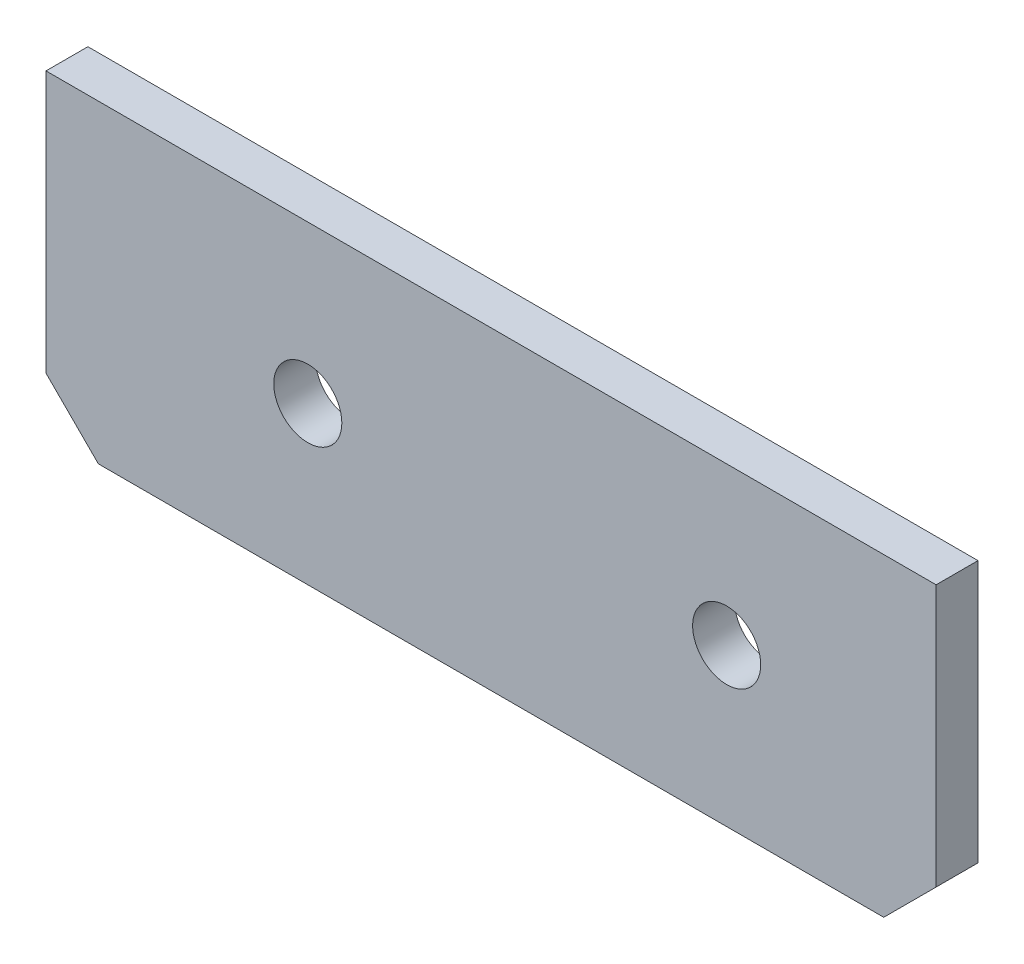
from build123d import *

# Parameters (mm, degrees)
EXTRUDE_1_DEPTH     = 8
SKETCH_2_R          = 6.5
CUT_EXTRUDE_1_DEPTH = 8


with BuildPart() as part:
    # 草图1 → 凸台-拉伸1 (new body)
    with BuildSketch(Plane.XY):
        Polygon((10, 0), (160, 0), (170, 10), (170, 60), (0, 60), (0, 10), align=None)
    extrude(amount=EXTRUDE_1_DEPTH)

    # 草图2 → 切除-拉伸1 (cut)
    with BuildSketch(Plane.XY.offset(8)):
        with Locations((50, 30)):
            Circle(SKETCH_2_R)
        with Locations((130, 30)):
            Circle(SKETCH_2_R)
    extrude(amount=-CUT_EXTRUDE_1_DEPTH, mode=Mode.SUBTRACT)


solid = part.part
